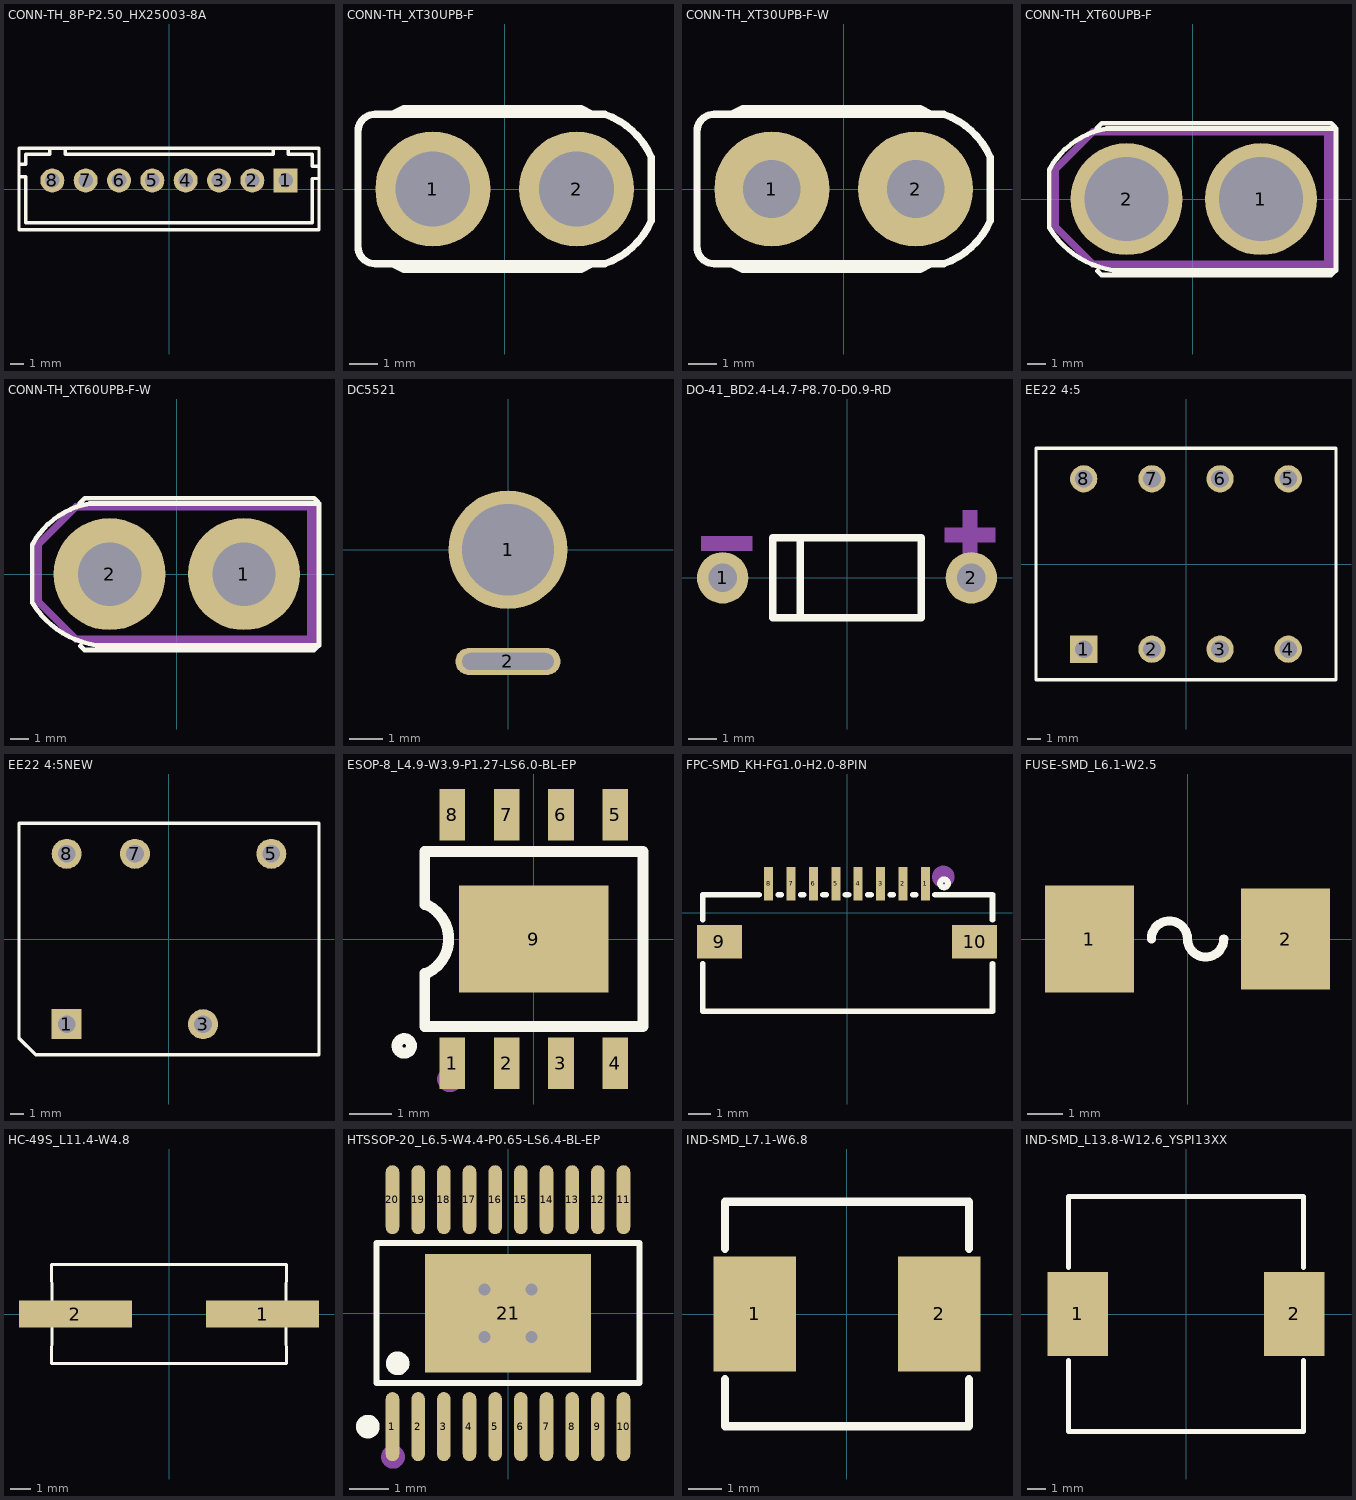
[diagram p0: the footprints below, top view; thin cyan lines are the x and y axes]
# Altium footprint library MISC84402-3.PcbLib: 74 footprints (part 2 of 5)
Each footprint in its own frame and in the unit in brackets; x right, y up, seen from the top. Pads: shape width x height; smd on the part's side, far side on the other; paste and mask are expansions set on the pad; w line width, h text height; cw(c..) or ccw(c..) is an arc to the next point about the centre after c.

## CONN-TH_8P-P2.50_HX25003-8A [mm]
pads (8):
  rect 1.8x1.8 hole 1.1: 1(8.75,0.646)
  round 1.8 hole 1.1: 2(6.25,0.646) 3(3.75,0.646) 4(1.25,0.646) 5(-1.25,0.646) 6(-3.75,0.646) 7(-6.25,0.646) 8(-8.75,0.646)
Top Overlay:
  lines w0.254: -11.25,0.915 -10.75,0.915 -10.75,-2.521 10.749,-2.521 10.749,0.786 11.249,0.786 ; -11.25,1.845 -10.75,1.845 -10.75,2.604 -8.944,2.604 -8.944,3.054 ; -7.8,2.604 7.8,2.604 ; -7.793,2.601 -7.793,3.05 ; 7.807,2.601 7.807,3.05 ; 8.943,2.604 10.749,2.604 10.749,1.715 11.249,1.715 ; 8.95,2.602 8.95,3.05 ; -11.25,-3.054 11.25,-3.054 11.25,3.046 -11.25,3.046 -11.25,-3.054

## CONN-TH_XT30UPB-F [mm]
pads (2):
  round 4 hole 2.6: 1(-2.5,0) 2(2.5,0)
Top Overlay:
  lines w0.254: -3.9,-2.6 -3.5,-2.8 2.65,-2.8 3.05,-2.6 ; -3.9,2.6 -3.5,2.8 2.65,2.8 3.05,2.6 ; -5.1,-2 ccw(c-4.5,-2) -4.5,-2.6 3.475,-2.6 ccw(c2.58,0) 5.1,-1.1 5.1,1.1 ccw(c2.58,0) 3.475,2.6 -4.5,2.6 ccw(c-4.5,2) -5.1,2 -5.1,-2

## CONN-TH_XT30UPB-F-W [mm]
pads (2):
  round 4 hole 2: 1(-2.5,0) 2(2.5,0)
Top Overlay:
  lines w0.254: -3.9,-2.6 -3.5,-2.8 2.65,-2.8 3.05,-2.6 ; -3.9,2.6 -3.5,2.8 2.65,2.8 3.05,2.6 ; -5.1,-2 ccw(c-4.5,-2) -4.5,-2.6 3.475,-2.6 ccw(c2.579,0) 5.1,-1.1 5.1,1.1 ccw(c2.579,0) 3.475,2.6 -4.5,2.6 ccw(c-4.5,2) -5.1,2 -5.1,-2

## CONN-TH_XT60UPB-F [mm]
pads (2):
  round 6 hole 4.5: 1(3.663,0) 2(-3.536,0)
Top Overlay:
  lines w0.254: -7.683,-1.524 -7.683,1.576 cw(c-3.873,-0.482) -4.625,3.783 7.683,3.783 7.683,-3.819 ; -7.668,-1.548 ccw(c-3.507,1.016) -4.283,-3.81 7.658,-3.81 ; -5.119,3.819 -4.874,4.064 -4.827,4.064 7.419,4.064 7.638,3.844 ; -5.099,-3.844 -4.88,-4.064 7.365,-4.064 7.413,-4.064 7.658,-3.819
Mechanical 15:
  region: -5.397,3.81 -7.556,1.651 -7.302,1.397 -5.143,3.556
  region: -7.556,-1.524 -5.397,-3.683 -5.143,-3.429 -7.302,-1.27
  region: -7.556,1.651 -7.556,-1.524 -7.175,-1.524 -7.175,1.651
  region: -5.397,3.81 7.556,3.81 7.556,3.429 -5.271,3.429
  region: -5.397,-3.683 -5.397,-3.302 7.556,-3.302 7.556,-3.683
  region: 7.556,3.429 7.556,-3.302 7.048,-3.302 7.048,3.429

## CONN-TH_XT60UPB-F-W [mm]
pads (2):
  round 6 hole 3.4: 1(3.6,0) 2(-3.6,0)
Top Overlay:
  lines w0.254: -7.747,-1.524 -7.747,1.576 cw(c-3.937,-0.482) -4.689,3.782 7.62,3.782 7.62,-3.819 ; -7.732,-1.548 ccw(c-3.57,1.016) -4.346,-3.81 7.595,-3.81 ; -5.183,3.819 -4.938,4.064 -4.89,4.064 7.355,4.064 7.575,3.844 ; -5.163,-3.844 -4.943,-4.064 7.302,-4.064 7.35,-4.064 7.595,-3.819
Mechanical 15:
  region: -5.461,3.81 -7.62,1.651 -7.366,1.397 -5.207,3.556
  region: -7.62,-1.524 -5.461,-3.683 -5.207,-3.429 -7.366,-1.27
  region: -7.62,1.651 -7.62,-1.524 -7.239,-1.524 -7.239,1.651
  region: -5.461,3.81 7.493,3.81 7.493,3.429 -5.334,3.429
  region: -5.461,-3.683 -5.461,-3.302 7.493,-3.302 7.493,-3.683
  region: 7.493,3.429 7.493,-3.302 6.985,-3.302 6.985,3.429

## DC5521 [mm]
pads (2):
  round 3.5 hole 2.7: 1(0,0)
  oval 3.1x0.8 hole 0.5 slot 2.7 at 0 deg: 2(0,-3.302)
Bottom Overlay:
  circle w0.254: c0,0 r4

## DO-41_BD2.4-L4.7-P8.70-D0.9-RD [mm]
pads (2):
  round 1.8 hole 1: 1(-4.35,0) 2(4.35,0)
Top Overlay:
  lines w0.254: -1.641,-1.4 -1.641,1.4 ; -2.6,-1.4 -2.6,1.4 2.6,1.4 2.6,-1.4 -2.6,-1.4
Mechanical 15:
  region: -5.102,1.451 -3.324,1.451 -3.324,0.943 -5.102,0.943
  region: 4.045,0.593 4.045,2.371 4.553,2.371 4.553,0.593
  region: 3.415,1.759 5.193,1.759 5.193,1.251 3.415,1.251

## EE22 4:5 [mm]
pads (8):
  rect 2x2 hole 1.3: 1(-7.5,-6.25)
  round 2 hole 1.3: 2(-2.5,-6.25) 3(2.5,-6.25) 4(7.5,-6.25) 5(7.5,6.25) 6(2.5,6.25) 7(-2.5,6.25) 8(-7.5,6.25)
Top Overlay:
  lines w0.254: -11,-8.5 11,-8.5 11,8.5 -11,8.5 -11,-8.5

## EE22 4:5NEW [mm]
pads (5):
  rect 2.2x2.2 hole 1.3: 1(-7.5,-6.25)
  round 2.2 hole 1.3: 3(2.5,-6.25) 5(7.5,6.25) 7(-2.5,6.25) 8(-7.5,6.25)
Top Overlay:
  lines w0.254: -11,-7.279 -11,-7.18 -11,8.5 11,8.5 11,-8.5 -9.779,-8.5 -11,-7.279

## ESOP-8_L4.9-W3.9-P1.27-LS6.0-BL-EP [mm]
pads (9):
  rect 0.6x1.2 smd: 1(-1.905,-2.908) 2(-0.635,-2.908) 3(0.635,-2.908) 4(1.905,-2.908) 5(1.905,2.908) 6(0.635,2.908) 7(-0.635,2.908) 8(-1.905,2.908)
  rect 3.5x2.5 smd: 9(0,0)
Top Overlay:
  circle w0.254: c-3.03,-2.5 r0.17
  lines w0.254: -2.55,-0.8 -2.55,-2.05 2.55,-2.05 2.55,2.05 -2.55,2.05 -2.55,0.8 ; -2.5,-0.8 ccw(c-2.875,0) -2.5,0.8
Mechanical 15:
  circle w0.3: c-1.96,-3.28 r0.15

## FPC-SMD_KH-FG1.0-H2.0-8PIN [mm]
pads (10):
  rect 0.4x1.5 smd: 1(3.5,1.3) 2(2.5,1.3) 3(1.5,1.3) 4(0.5,1.3) 5(-0.5,1.3) 6(-1.5,1.3) 7(-2.5,1.3) 8(-3.5,1.3)
  rect 2x1.5 smd: 9(-5.7,-1.3) 10(5.7,-1.3)
Top Overlay:
  circle w0.254: c4.335,1.308 r0.18
  lines w0.254: -6.45,-2.281 -6.45,-4.4 6.5,-4.4 6.5,-2.281 ; -6.45,-0.319 -6.45,0.8 -3.931,0.8 ; -3.069,0.8 -2.931,0.8 ; -2.069,0.8 -1.931,0.8 ; -1.069,0.8 -0.931,0.8 ; -0.069,0.8 0.069,0.8 ; 0.931,0.8 1.069,0.8 ; 1.931,0.8 2.069,0.8 ; 2.931,0.8 3.069,0.8 ; 3.931,0.8 6.5,0.8 6.5,-0.319
Mechanical 15:
  circle w0.5: c4.3,1.6 r0.25

## FUSE-SMD_L6.1-W2.5 [mm]
pads (2):
  rect 2.5x3 smd: 1(-2.75,0)
  rect 2.5x2.83 smd: 2(2.75,0)
Top Overlay:
  lines w0.254: -1.016,0 cw(c-0.508,0) 0,0 ccw(c0.508,0) 1.016,0

## HC-49S_L11.4-W4.8 [mm]
pads (2):
  rect 5.5x1.3 smd: 1(4.553,0) 2(-4.553,0)
Top Overlay:
  lines w0.152: -5.715,-2.413 5.715,-2.413 ; -5.715,-2.413 -5.7,-0.662 -5.715,-2.413 ; -5.715,-2.413 5.715,-2.413 ; -5.715,2.413 -5.7,0.662 -5.715,2.413 ; -5.715,2.413 5.715,2.413 ; -5.715,2.413 5.715,2.413 ; 5.715,-2.413 5.7,-0.662 5.715,-2.413 ; 5.715,2.413 5.7,0.662 5.715,2.413

## HTSSOP-20_L6.5-W4.4-P0.65-LS6.4-BL-EP [mm]
pads (21):
  oval 0.343x1.747 smd: 1(-2.925,-2.873) 2(-2.275,-2.873) 3(-1.625,-2.873) 4(-0.975,-2.873) 5(-0.325,-2.873) 6(0.325,-2.873) 7(0.975,-2.873) 8(1.625,-2.873) 9(2.275,-2.873) 10(2.925,-2.873) 11(2.925,2.873) 12(2.275,2.873) 13(1.625,2.873) 14(0.975,2.873) 15(0.325,2.873) 16(-0.325,2.873) 17(-0.975,2.873) 18(-1.625,2.873) 19(-2.275,2.873) 20(-2.925,2.873)
  rect 4.2x3 smd: 21(0,0)
via 0.6,0.6 diameter 0.61 hole 0.305
via -0.6,0.6 diameter 0.61 hole 0.305
via -0.6,-0.6 diameter 0.61 hole 0.305
via 0.6,-0.6 diameter 0.61 hole 0.305
Top Overlay:
  circle w0.3: c-3.549,-2.873 r0.15
  circle w0.3: c-2.794,-1.27 r0.15
  lines w0.152: -3.326,-1.771 -3.326,1.771 3.326,1.771 3.326,-1.771 -3.326,-1.771
Mechanical 15:
  circle w0.3: c-2.912,-3.638 r0.15

## IND-SMD_L7.1-W6.8 [mm]
pads (2):
  rect 2.5x3.5 smd: 1(-2.8,0) 2(2.8,0)
Top Overlay:
  lines w0.254: -3.7,-1.981 -3.7,-3.4 3.7,-3.4 3.7,-1.981 ; -3.7,1.981 -3.7,3.4 3.7,3.4 3.7,1.981

## IND-SMD_L13.8-W12.6_YSPI13XX [mm]
pads (2):
  rect 3.25x4.5 smd: 1(-5.8,0) 2(5.8,0)
Top Overlay:
  lines w0.254: -6.3,-2.481 -6.3,-6.3 6.3,-6.3 6.3,-2.481 ; -6.3,2.481 -6.3,6.3 6.3,6.3 6.3,2.481